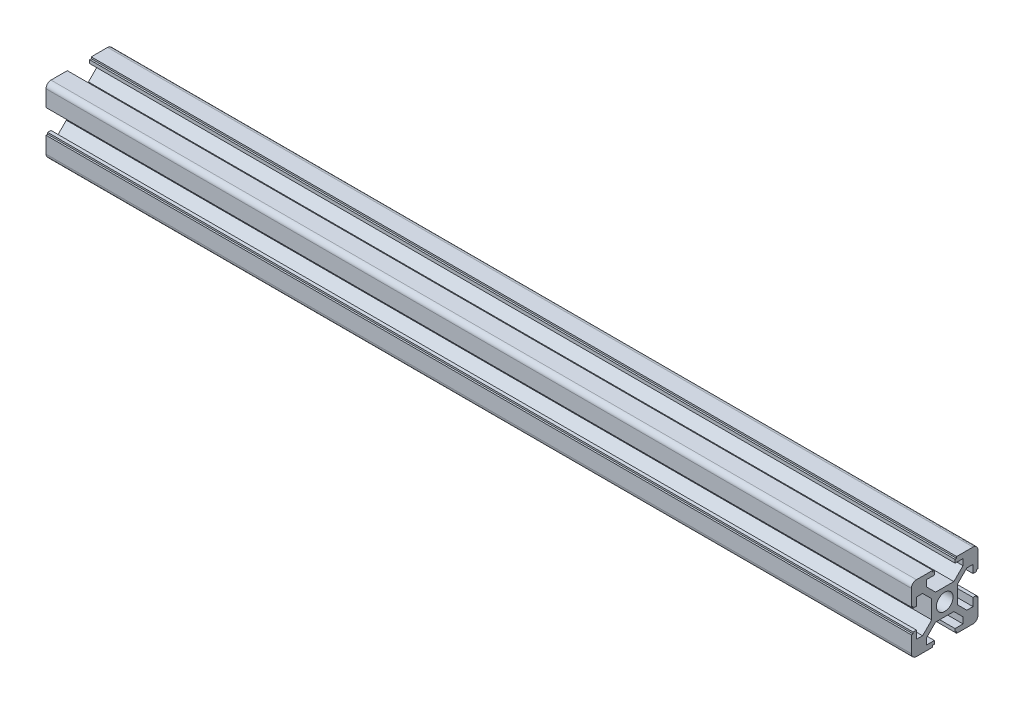
from build123d import *

# Parameters (mm, degrees)
SKETCH1_R                = 2.5
F_20_X_20_X_R1_5_1_DEPTH = 260


with BuildPart() as part:
    # Sketch1 → 工业铝型材 20 X 20 X R1.5(1) (new body)
    with BuildSketch(Plane.YZ):
        with BuildLine():
            Line((-3.6, 10), (-3.6, 9.5))
            Line((-3.6, 9.5), (-3.1, 9.5))
            Line((-3.1, 9.5), (-3.1, 8.5))
            Line((-3.1, 8.5), (-5.5, 8.5))
            Line((-5.5, 8.5), (-5.5, 6.65))
            Line((-5.5, 6.65), (-2.75, 3.9))
            Line((-2.75, 3.9), (2.75, 3.9))
            Line((2.75, 3.9), (5.5, 6.65))
            Line((5.5, 6.65), (5.5, 8.5))
            Line((5.5, 8.5), (3.1, 8.5))
            Line((3.1, 8.5), (3.1, 9.5))
            Line((3.1, 9.5), (3.6, 9.5))
            Line((3.6, 9.5), (3.6, 10))
            Line((3.6, 10), (8.5, 10))
            ThreePointArc((8.5, 10), (9.560660172, 9.560660172), (10, 8.5))
            Line((10, 8.5), (10, 3.6))
            Line((10, 3.6), (9.5, 3.6))
            Line((9.5, 3.6), (9.5, 3.1))
            Line((9.5, 3.1), (8.5, 3.1))
            Line((8.5, 3.1), (8.5, 5.5))
            Line((8.5, 5.5), (6.65, 5.5))
            Line((6.65, 5.5), (3.9, 2.75))
            Line((3.9, 2.75), (3.9, -2.75))
            Line((3.9, -2.75), (6.65, -5.5))
            Line((6.65, -5.5), (8.5, -5.5))
            Line((8.5, -5.5), (8.5, -3.1))
            Line((8.5, -3.1), (9.5, -3.1))
            Line((9.5, -3.1), (9.5, -3.6))
            Line((9.5, -3.6), (10, -3.6))
            Line((10, -3.6), (10, -8.5))
            ThreePointArc((10, -8.5), (9.560660172, -9.560660172), (8.5, -10))
            Line((8.5, -10), (3.6, -10))
            Line((3.6, -10), (3.6, -9.5))
            Line((3.6, -9.5), (3.1, -9.5))
            Line((3.1, -9.5), (3.1, -8.5))
            Line((3.1, -8.5), (5.5, -8.5))
            Line((5.5, -8.5), (5.5, -6.65))
            Line((5.5, -6.65), (2.75, -3.9))
            Line((2.75, -3.9), (-2.75, -3.9))
            Line((-2.75, -3.9), (-5.5, -6.65))
            Line((-5.5, -6.65), (-5.5, -8.5))
            Line((-5.5, -8.5), (-3.1, -8.5))
            Line((-3.1, -8.5), (-3.1, -9.5))
            Line((-3.1, -9.5), (-3.6, -9.5))
            Line((-3.6, -9.5), (-3.6, -10))
            Line((-3.6, -10), (-8.5, -10))
            ThreePointArc((-8.5, -10), (-9.560660172, -9.560660172), (-10, -8.5))
            Line((-10, -8.5), (-10, -3.6))
            Line((-10, -3.6), (-9.5, -3.6))
            Line((-9.5, -3.6), (-9.5, -3.1))
            Line((-9.5, -3.1), (-8.5, -3.1))
            Line((-8.5, -3.1), (-8.5, -5.5))
            Line((-8.5, -5.5), (-6.65, -5.5))
            Line((-6.65, -5.5), (-3.9, -2.75))
            Line((-3.9, -2.75), (-3.9, 2.75))
            Line((-3.9, 2.75), (-6.65, 5.5))
            Line((-6.65, 5.5), (-8.5, 5.5))
            Line((-8.5, 5.5), (-8.5, 3.1))
            Line((-8.5, 3.1), (-9.5, 3.1))
            Line((-9.5, 3.1), (-9.5, 3.6))
            Line((-9.5, 3.6), (-10, 3.6))
            Line((-10, 3.6), (-10, 8.5))
            ThreePointArc((-10, 8.5), (-9.560660172, 9.560660172), (-8.5, 10))
            Line((-8.5, 10), (-3.6, 10))
        make_face()
        Circle(SKETCH1_R, mode=Mode.SUBTRACT)
    extrude(amount=F_20_X_20_X_R1_5_1_DEPTH)


solid = part.part
